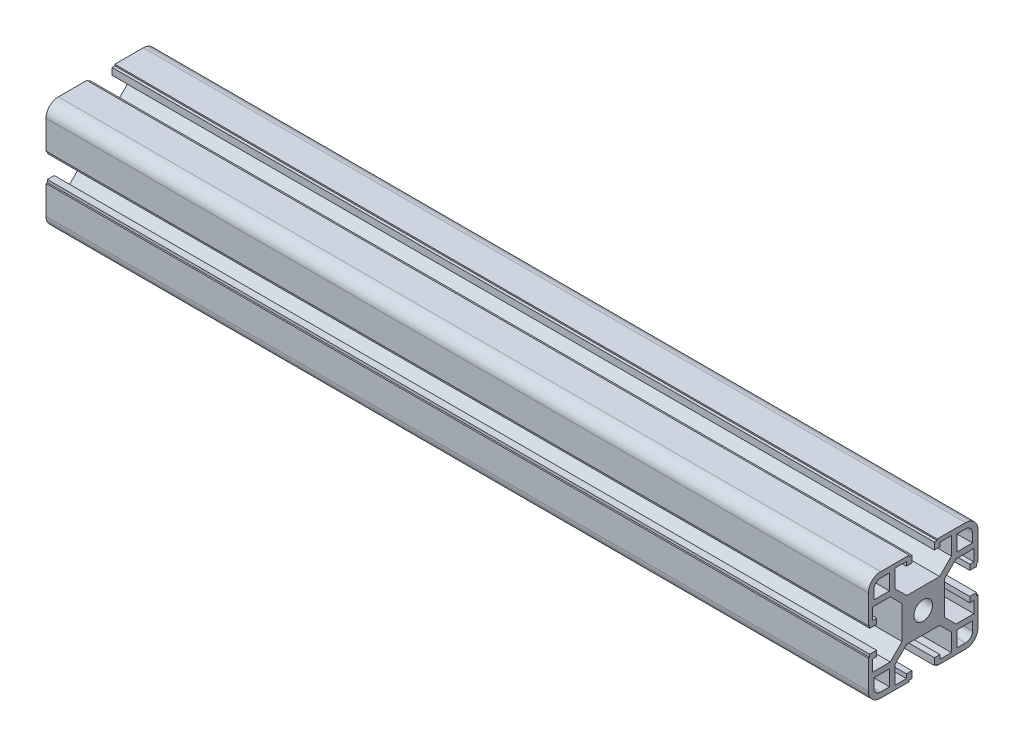
SolidWorks part; units mm, degrees
ref_plane "Front Plane" through (0, 0, 0) normal (0, 0, 1) x (1, 0, 0)
ref_plane "Top Plane" through (0, 0, 0) normal (0, 1, 0) x (1, 0, 0)
ref_plane "Right Plane" through (0, 0, 0) normal (1, 0, 0) x (0, 0, -1)
sketch "草图1" plane through (0, 0, 0) normal (0, 0, 1) x (1, 0, 0)
  line L0 (-984.975, 0) -> (-684.975, 0)
  dimension "D1" = 300
other "Aluminium profile 40 X 40B X R4.5(1)"
ref_plane "Plane1" through (-984.975, 0, 0) normal (1, 0, 0) x (0, 1, 0)
sketch "Sketch1" plane through (-984.975, 0, 0) normal (1, 0, 0) x (0, 1, 0)
  line L0 (-5.1, 20) -> (-5.1, 19.5)
  line L1 (-5.1, 19.5) -> (-4.1, 19.5)
  line L2 (-4.1, 19.5) -> (-4.1, 17)
  line L3 (-6.1, 18.5) -> (-10.3, 18.5)
  line L4 (-15.5, -20) -> (-5.1, -20)
  line L5 (-20, -15.5) -> (-20, -5.1)
  line L6 (15.5, 20) -> (5.1, 20)
  line L7 (20, 15.5) -> (20, 5.1)
  line L8 (0, 14.8756) -> (0, 0) construction
  line L9 (0, 0) -> (14.1675, 0) construction
  line L10 (-10.3, 18.5) -> (-10.3, 12)
  line L11 (-10.3, 12) -> (-6, 7.7)
  line L12 (-6, 7.7) -> (6, 7.7)
  line L13 (10.3, 12) -> (6, 7.7)
  line L14 (10.3, 18.5) -> (10.3, 12)
  line L15 (6.1, 18.5) -> (10.3, 18.5)
  line L16 (4.1, 19.5) -> (4.1, 17)
  line L17 (5.1, 19.5) -> (4.1, 19.5)
  line L18 (5.1, 20) -> (5.1, 19.5)
  line L19 (-5.1, 20) -> (-15.5, 20)
  line L20 (20, 5.1) -> (19.5, 5.1)
  line L21 (12.3, 18) -> (15.5, 18)
  line L22 (12.3, 18) -> (12.3, 12.3)
  line L23 (12.3, 12.3) -> (18, 12.3)
  line L24 (18, 15.5) -> (18, 12.3)
  line L25 (19.5, 5.1) -> (19.5, 4.1)
  line L26 (19.5, 4.1) -> (17, 4.1)
  line L27 (17, 6.1) -> (17, 4.1)
  line L28 (18.5, 6.1) -> (17, 6.1)
  line L29 (18.5, 6.1) -> (18.5, 10.3)
  line L30 (18.5, 10.3) -> (12, 10.3)
  line L31 (12, 10.3) -> (7.7, 6)
  line L32 (7.7, 6) -> (7.7, -6)
  line L33 (12, -10.3) -> (7.7, -6)
  line L34 (18.5, -10.3) -> (12, -10.3)
  line L35 (18.5, -6.1) -> (18.5, -10.3)
  line L36 (18.5, -6.1) -> (17, -6.1)
  line L37 (17, -4.1) -> (17, -6.1)
  line L38 (19.5, -4.1) -> (17, -4.1)
  line L39 (19.5, -5.1) -> (19.5, -4.1)
  line L40 (20, -5.1) -> (19.5, -5.1)
  line L41 (5.1, -20) -> (5.1, -19.5)
  line L42 (5.1, -19.5) -> (4.1, -19.5)
  line L43 (4.1, -19.5) -> (4.1, -17)
  line L44 (6.1, -17) -> (4.1, -17)
  line L45 (6.1, -18.5) -> (6.1, -17)
  line L46 (6.1, -18.5) -> (10.3, -18.5)
  line L47 (10.3, -18.5) -> (10.3, -12)
  line L48 (10.3, -12) -> (6, -7.7)
  line L49 (6, -7.7) -> (-6, -7.7)
  line L50 (-10.3, -12) -> (-6, -7.7)
  line L51 (-10.3, -18.5) -> (-10.3, -12)
  line L52 (-6.1, -18.5) -> (-10.3, -18.5)
  line L53 (-6.1, -18.5) -> (-6.1, -17)
  line L54 (-4.1, -17) -> (-6.1, -17)
  line L55 (-4.1, -19.5) -> (-4.1, -17)
  line L56 (-5.1, -19.5) -> (-4.1, -19.5)
  line L57 (-5.1, -20) -> (-5.1, -19.5)
  line L58 (-20, -5.1) -> (-19.5, -5.1)
  line L59 (5.1, -20) -> (15.5, -20)
  line L60 (-20, 5.1) -> (-20, 15.5)
  line L61 (-19.5, -5.1) -> (-19.5, -4.1)
  line L62 (-6.1, 18.5) -> (-6.1, 17)
  line L63 (-6.1, 17) -> (-4.1, 17)
  line L64 (6.1, 18.5) -> (6.1, 17)
  line L65 (4.1, 17) -> (6.1, 17)
  line L66 (-19.5, -4.1) -> (-17, -4.1)
  line L67 (-15.5, 18) -> (-12.3, 18)
  line L68 (-18, 15.5) -> (-18, 12.3)
  line L69 (-18, 12.3) -> (-12.3, 12.3)
  line L70 (-12.3, 18) -> (-12.3, 12.3)
  line L71 (-17, -6.1) -> (-17, -4.1)
  line L72 (-18.5, -6.1) -> (-17, -6.1)
  line L73 (-18.5, -6.1) -> (-18.5, -10.3)
  line L74 (-18.5, -10.3) -> (-12, -10.3)
  line L75 (-12, -10.3) -> (-7.7, -6)
  line L76 (-7.7, -6) -> (-7.7, 6)
  line L77 (-12, 10.3) -> (-7.7, 6)
  line L78 (-18.5, 10.3) -> (-12, 10.3)
  line L79 (-18.5, 6.1) -> (-18.5, 10.3)
  line L80 (-18.5, 6.1) -> (-17, 6.1)
  line L81 (-17, 4.1) -> (-17, 6.1)
  line L82 (-19.5, 4.1) -> (-17, 4.1)
  line L83 (-19.5, 5.1) -> (-19.5, 4.1)
  line L84 (-20, 5.1) -> (-19.5, 5.1)
  line L85 (20, -5.1) -> (20, -15.5)
  line L87 (-18, -12.3) -> (-12.3, -12.3)
  line L88 (-18, -12.3) -> (-18, -15.5)
  line L89 (-15.5, -18) -> (-12.3, -18)
  line L90 (-12.3, -12.3) -> (-12.3, -18)
  line L91 (12.3, -12.3) -> (18, -12.3)
  line L92 (12.3, -12.3) -> (12.3, -18)
  line L93 (12.3, -18) -> (15.5, -18)
  line L94 (18, -12.3) -> (18, -15.5)
  circle A0 centre (0, 0) radius 3.4
  arc A1 (-20, 15.5) -> (-15.5, 20) centre (-15.5, 15.5) cw
  arc A2 (20, 15.5) -> (15.5, 20) centre (15.5, 15.5) ccw
  arc A3 (-15.5, -20) -> (-20, -15.5) centre (-15.5, -15.5) cw
  arc A4 (15.5, -20) -> (20, -15.5) centre (15.5, -15.5) ccw
  arc A5 (-15.5, 18) -> (-18, 15.5) centre (-15.5, 15.5) ccw
  arc A6 (18, 15.5) -> (15.5, 18) centre (15.5, 15.5) ccw
  arc A7 (18, -15.5) -> (15.5, -18) centre (15.5, -15.5) cw
  arc A8 (-18, -15.5) -> (-15.5, -18) centre (-15.5, -15.5) ccw
  point P2 (0, 10)
  point P4 (0, 0)
  point P5 (-20, -20)
  point P6 (20, -20)
  point P7 (20, 20)
  point P8 (-20, 20)
  point P36 (-20, 20)
  point P39 (20, 20)
  point P121 (0, 0)
  dimension "D1" = 20.6
  dimension "D2" = 40
  dimension "D3" = 8.2
  dimension "D4" = 10.2
  dimension "D5" = 12.3
  dimension "D6" = 6.8
  dimension "D7" = 4.5
  dimension "D8" = 45
  dimension "D12" = 2
  dimension "D13" = 5.7
  dimension "D14" = 2
  dimension "D18" = 2.5
  dimension "D19" = 2.5
  dimension "D15" = 2.5
  dimension "D9" = 0.5
  dimension "D10" = 1.5
  dimension "D11" = 12
  dimension "D16" = 3
  dimension "D17" = 2
  dimension "D20" = 2
  dimension "D21" = 2
